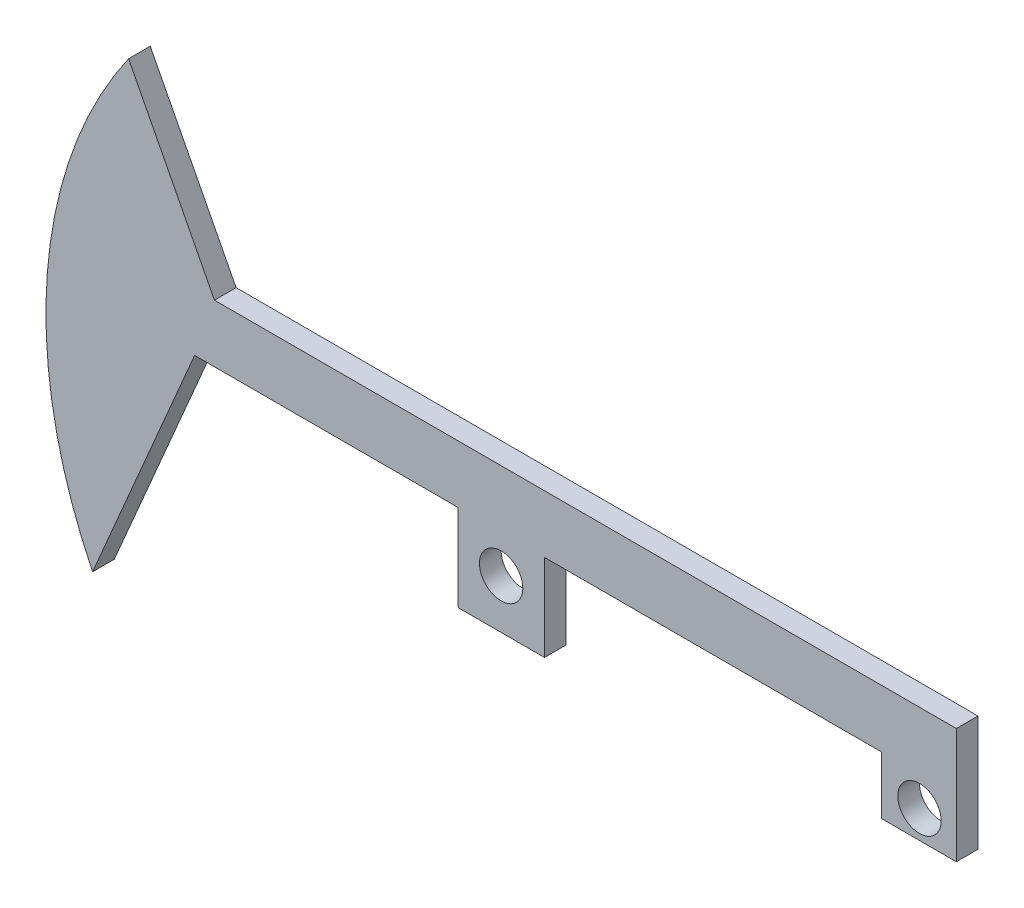
SolidWorks part; units mm, degrees
ref_plane "Front Plane" through (0, 0, 0) normal (0, 0, 1) x (1, 0, 0)
ref_plane "Top Plane" through (0, 0, 0) normal (0, 1, 0) x (1, 0, 0)
ref_plane "Right Plane" through (0, 0, 0) normal (1, 0, 0) x (0, 0, -1)
sketch "Sketch1" plane through (0, 0, 0) normal (0, 0, 1) x (1, 0, 0)
  line L0 (-1718.6749, 1206.7132) -> (-1322.5712, 440.1666)
  line L1 (-1322.5712, 440.1666) -> (2100, 440.1666)
  line L2 (-1884.7376, -926.1557) -> (-1413.9528, 173.8838)
  line L3 (-1413.9528, 173.8838) -> (-200, 173.8838)
  line L4 (1098.892, 173.8838) -> (1753.8949, 173.8838)
  line L5 (2100, 173.8838) -> (2100, 440.1666)
  line L6 (2100, 440.1666) -> (2102.8172, 426.3934)
  line L7 (1753.8949, 173.8838) -> (1753.8949, -92.399)
  line L8 (1753.8949, -92.399) -> (2100, -92.399)
  line L9 (2100, -92.399) -> (2100, 173.8838)
  line L10 (-200, 173.8838) -> (-200, -226.1162)
  line L11 (-200, -226.1162) -> (200, -226.1162)
  line L12 (200, -226.1162) -> (200, 173.8838)
  line L13 (200, 173.8838) -> (1098.892, 173.8838)
  arc A0 (-1718.6749, 1206.7132) -> (-1884.7376, -926.1557) centre (0, 0) ccw
  dimension "D1" = 4200
  dimension "D3" = 400
  dimension "D2" = 2100
  dimension "D4" = 400
  dimension "D5" = 200
extrude "Boss-Extrude1" add sketch "Sketch1" along normal blind 100 contours L1 L0 A0 L2 L3 L10 L11 L12 L13 L4 L7 L8 L9 L5
sketch "Sketch2" plane through (0, 0, 100) normal (0, 0, 1) x (1, 0, 0)
  circle A0 centre (1930.0376, 35.7543) radius 100
  circle A1 centre (0, 0) radius 100
  dimension "D1" = 200
  dimension "D2" = 200
extrude "Cut-Extrude1" cut sketch "Sketch2" against normal blind 100
